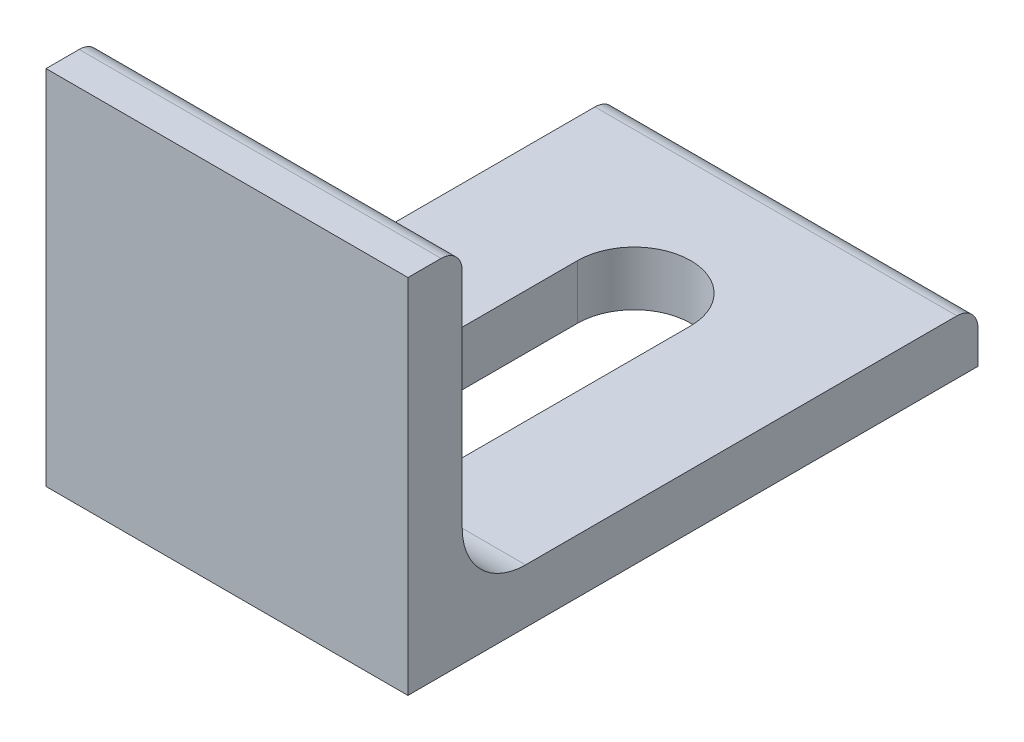
from build123d import *

# Parameters (mm, degrees)
HOT_ROLLED_UNEQUAL_ANGLE_GB_T_706_2008_6_DEPTH = 40
CUT_EXTRUDE1_DEPTH                             = 10


with BuildPart() as part:
    # Sketch1 → Hot-rolled unequal angle GB∕T 706-2008 63 X 40 X 6 (1) (new body)
    with BuildSketch(Plane(origin=(220, 114, 0), x_dir=(0, 1, 0), z_dir=(-1, 0, 0))):
        with BuildLine():
            Line((0, 0), (0, 63))
            Line((0, 63), (3.666666667, 63))
            ThreePointArc((3.666666667, 63), (5.316582489, 62.316582489), (6, 60.666666667))
            Line((6, 60.666666667), (6, 13))
            ThreePointArc((6, 13), (8.050252532, 8.050252532), (13, 6))
            Line((13, 6), (37.666666667, 6))
            ThreePointArc((37.666666667, 6), (39.316582489, 5.316582489), (40, 3.666666667))
            Line((40, 3.666666667), (40, 0))
            Line((40, 0), (0, 0))
        make_face()
    extrude(amount=HOT_ROLLED_UNEQUAL_ANGLE_GB_T_706_2008_6_DEPTH)

    # Sketch2 → Cut-Extrude1 (cut)
    with BuildSketch(Plane(origin=(0, 120, 0), x_dir=(1, 0, 0), z_dir=(0, 1, 0))):
        with BuildLine():
            Line((206.25, 45), (206.25, 20))
            ThreePointArc((206.25, 20), (200, 13.75), (193.75, 20))
            Line((193.75, 20), (193.75, 45))
            ThreePointArc((193.75, 45), (200, 51.25), (206.25, 45))
        make_face()
    extrude(amount=-CUT_EXTRUDE1_DEPTH, mode=Mode.SUBTRACT)


solid = part.part
